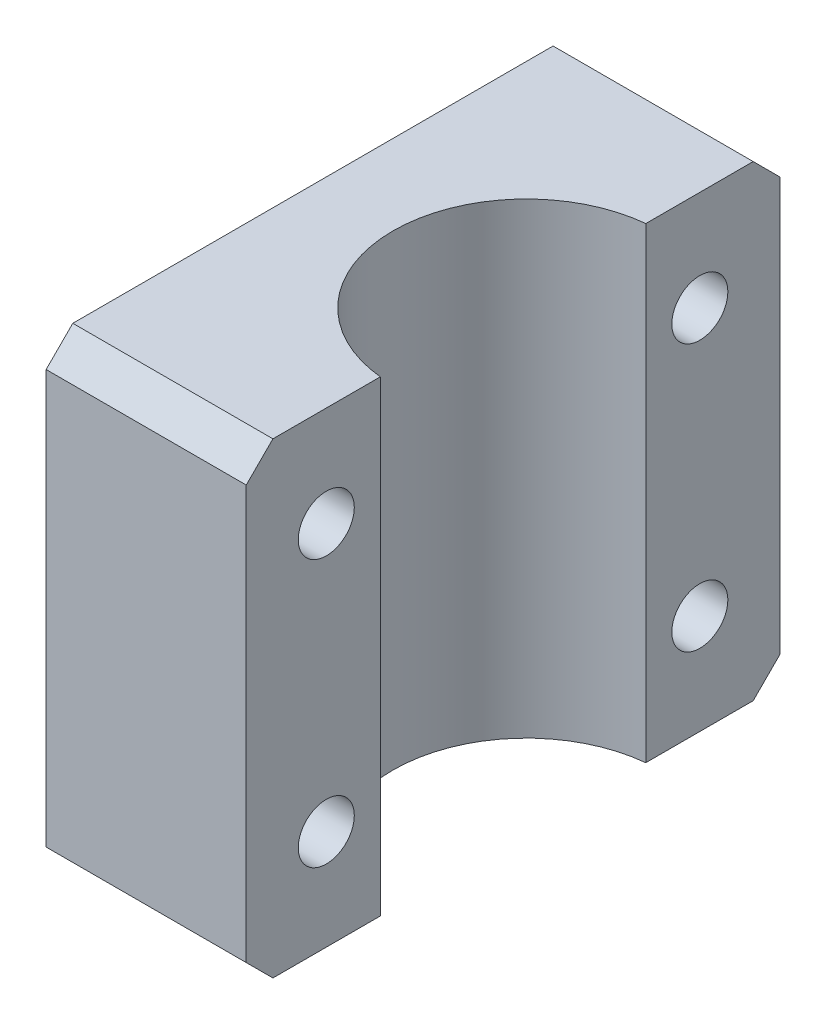
from build123d import *

# Parameters (mm, degrees)
EXTRUDE_1_DEPTH    = 17.5
CHAMFER_1_SIZE     = 2
HOLE_WIZARD_M5_1_D = 4.2


with BuildPart() as part:
    # 草图1 → 凸台-拉伸1 (new, symmetric)
    with BuildSketch(Plane(origin=(0, 0, 0), x_dir=(1, 0, 0), z_dir=(0, 1, 0))):
        with BuildLine():
            Line((7.5, 9.949874371), (7.5, 20))
            Line((7.5, 20), (-7.5, 20))
            Line((-7.5, 20), (-7.5, -20))
            Line((-7.5, -20), (7.5, -20))
            Line((7.5, -20), (7.5, -9.949874371))
            ThreePointArc((7.5, -9.949874371), (-1.5, 0), (7.5, 9.949874371))
        make_face()
    extrude(amount=EXTRUDE_1_DEPTH, both=True)

    # 倒角1
    chamfer_1_edges = [part.edges().sort_by_distance(p)[0] for p in [
        (0, 17.5, 20),
        (0, 17.5, -20),
        (0, -17.5, 20),
        (0, -17.5, -20),
    ]]
    chamfer(chamfer_1_edges, length=CHAMFER_1_SIZE)

    # M5 螺纹孔1 (through all)
    with Locations(Plane(origin=(7.5, 0, 0), x_dir=(0, 0, -1), z_dir=(1, 0, 0))):
        with Locations((-14, 10), (14, 10), (14, -10), (-14, -10)):
            Hole(HOLE_WIZARD_M5_1_D / 2)


solid = part.part
